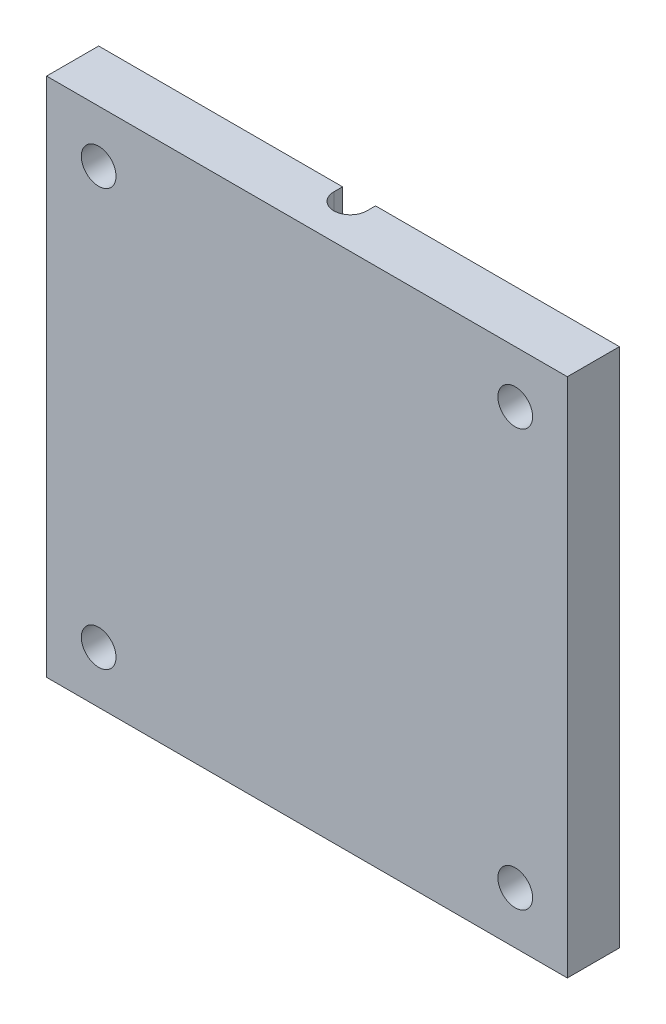
from build123d import *

# Parameters (mm, degrees)
SKETCH1_W           = 30
SKETCH1_H           = 30
BOSS_EXTRUDE1_DEPTH = 3
SKETCH2_R           = 1
CUT_EXTRUDE1_DEPTH  = 19
CUT_EXTRUDE2_DEPTH  = 42


with BuildPart() as part:
    # Sketch1 → Boss-Extrude1 (new body)
    with BuildSketch(Plane.XY):
        Rectangle(SKETCH1_W, SKETCH1_H)
    extrude(amount=BOSS_EXTRUDE1_DEPTH)

    # Sketch2 → Cut-Extrude1 (cut)
    with BuildSketch(Plane.XY.offset(3)):
        with Locations((-12, 12)):
            Circle(SKETCH2_R)
        with Locations((12, 12)):
            Circle(SKETCH2_R)
        with Locations((12, -12)):
            Circle(SKETCH2_R)
        with Locations((-12, -12)):
            Circle(SKETCH2_R)
    extrude(amount=-CUT_EXTRUDE1_DEPTH, mode=Mode.SUBTRACT)

    # Sketch3 → Cut-Extrude2 (cut)
    with BuildSketch(Plane.XZ.offset(15)):
        with BuildLine():
            Line((0.95, 0.5), (0.95, 0))
            Line((0.95, 0), (-0.95, 0))
            Line((-0.95, 0), (-0.95, 0.5))
            ThreePointArc((-0.95, 0.5), (0, 1.45), (0.95, 0.5))
        make_face()
    extrude(amount=-CUT_EXTRUDE2_DEPTH, mode=Mode.SUBTRACT)


solid = part.part
